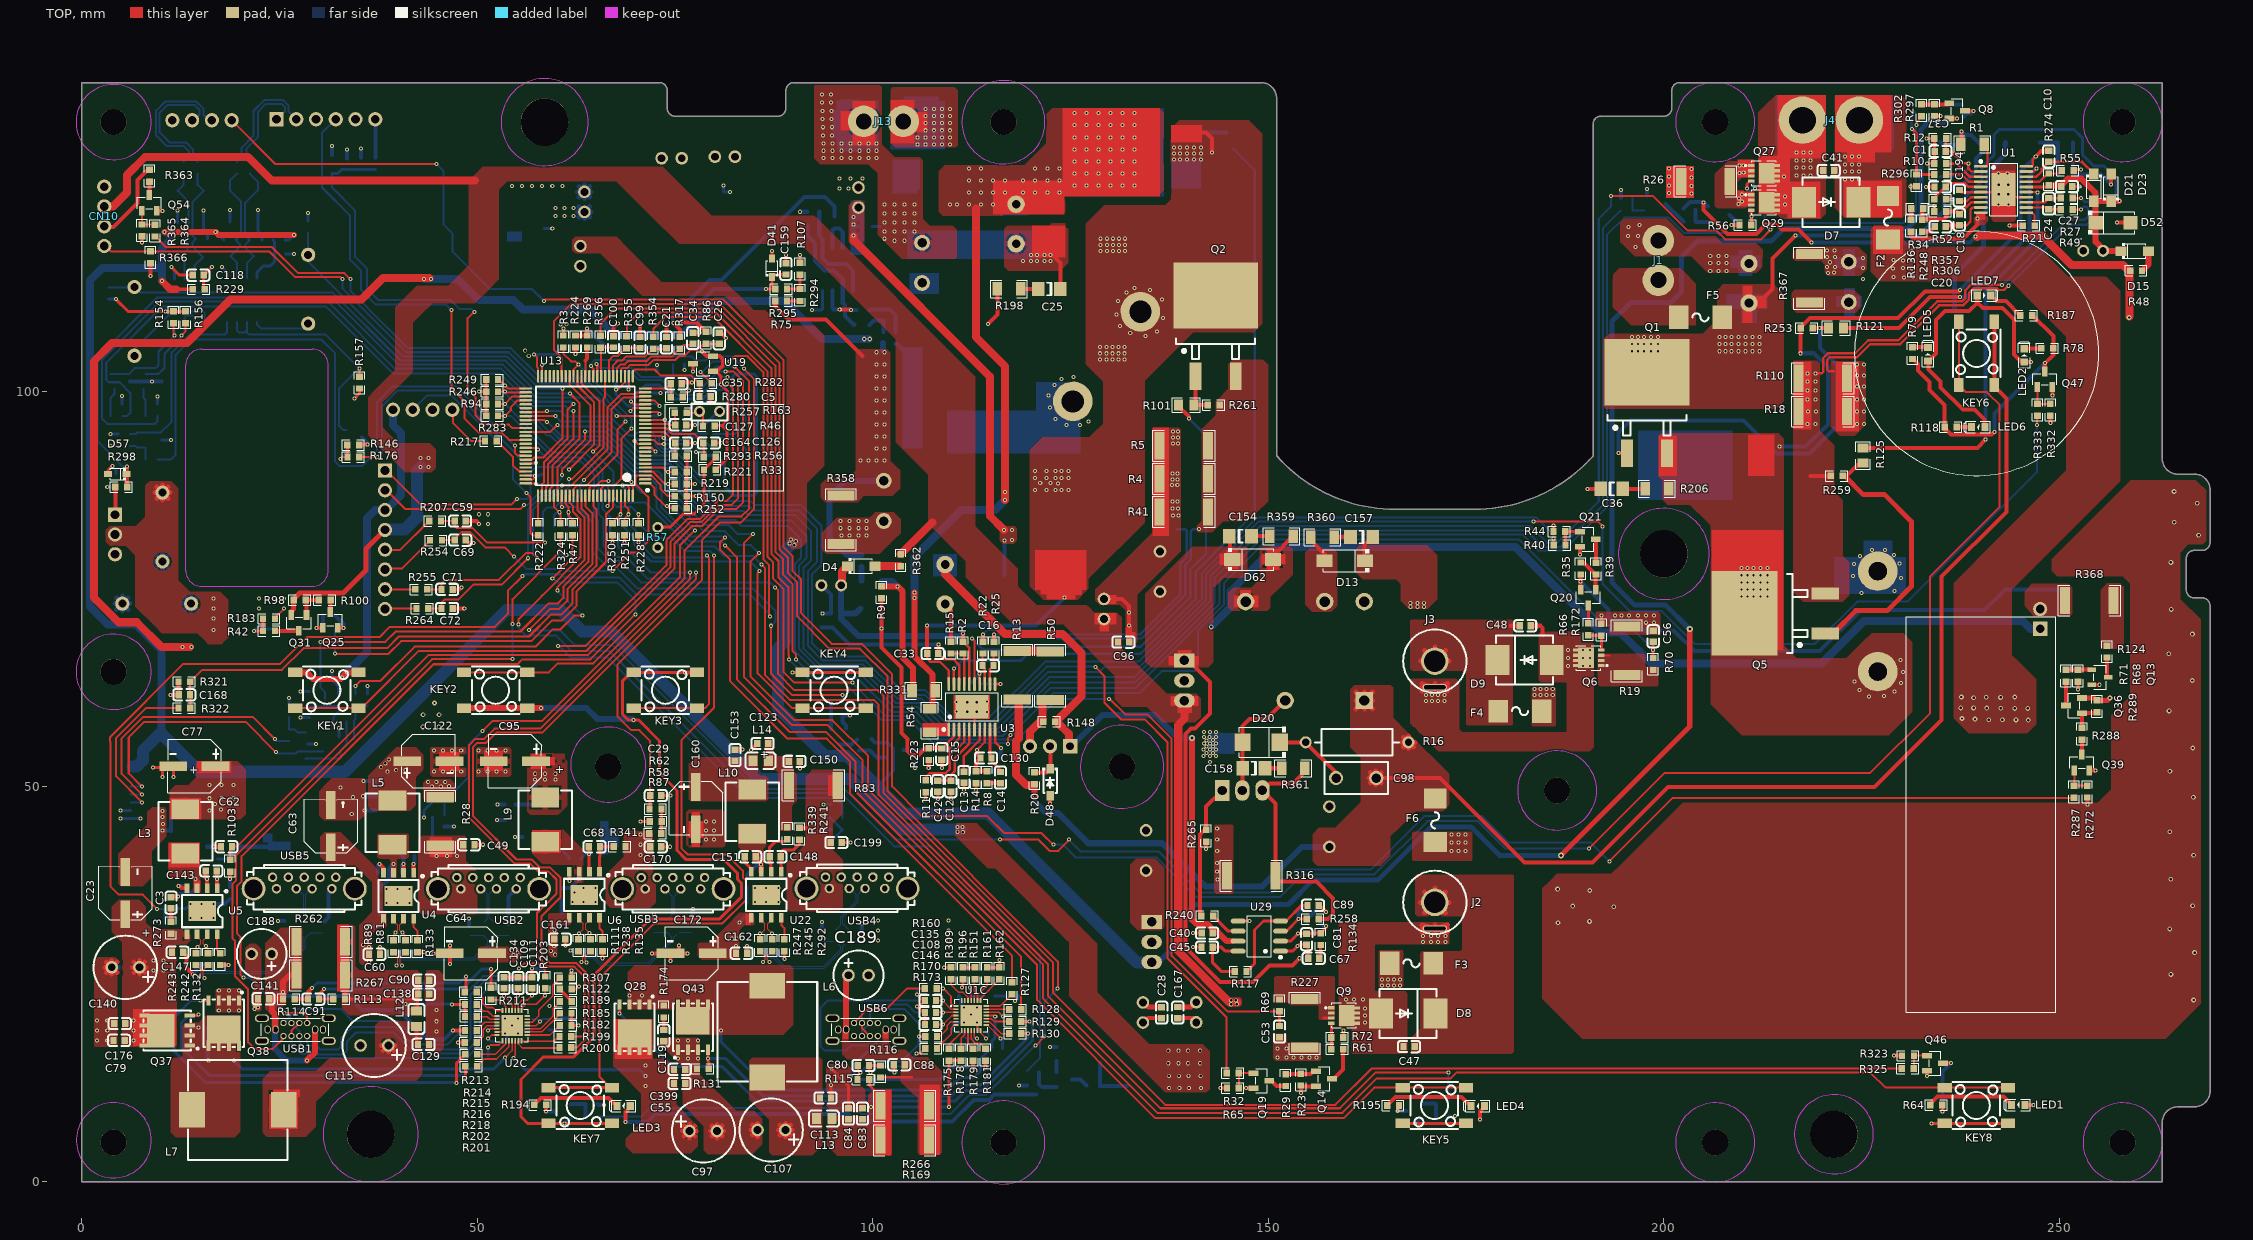
[diagram p0: TOP view]
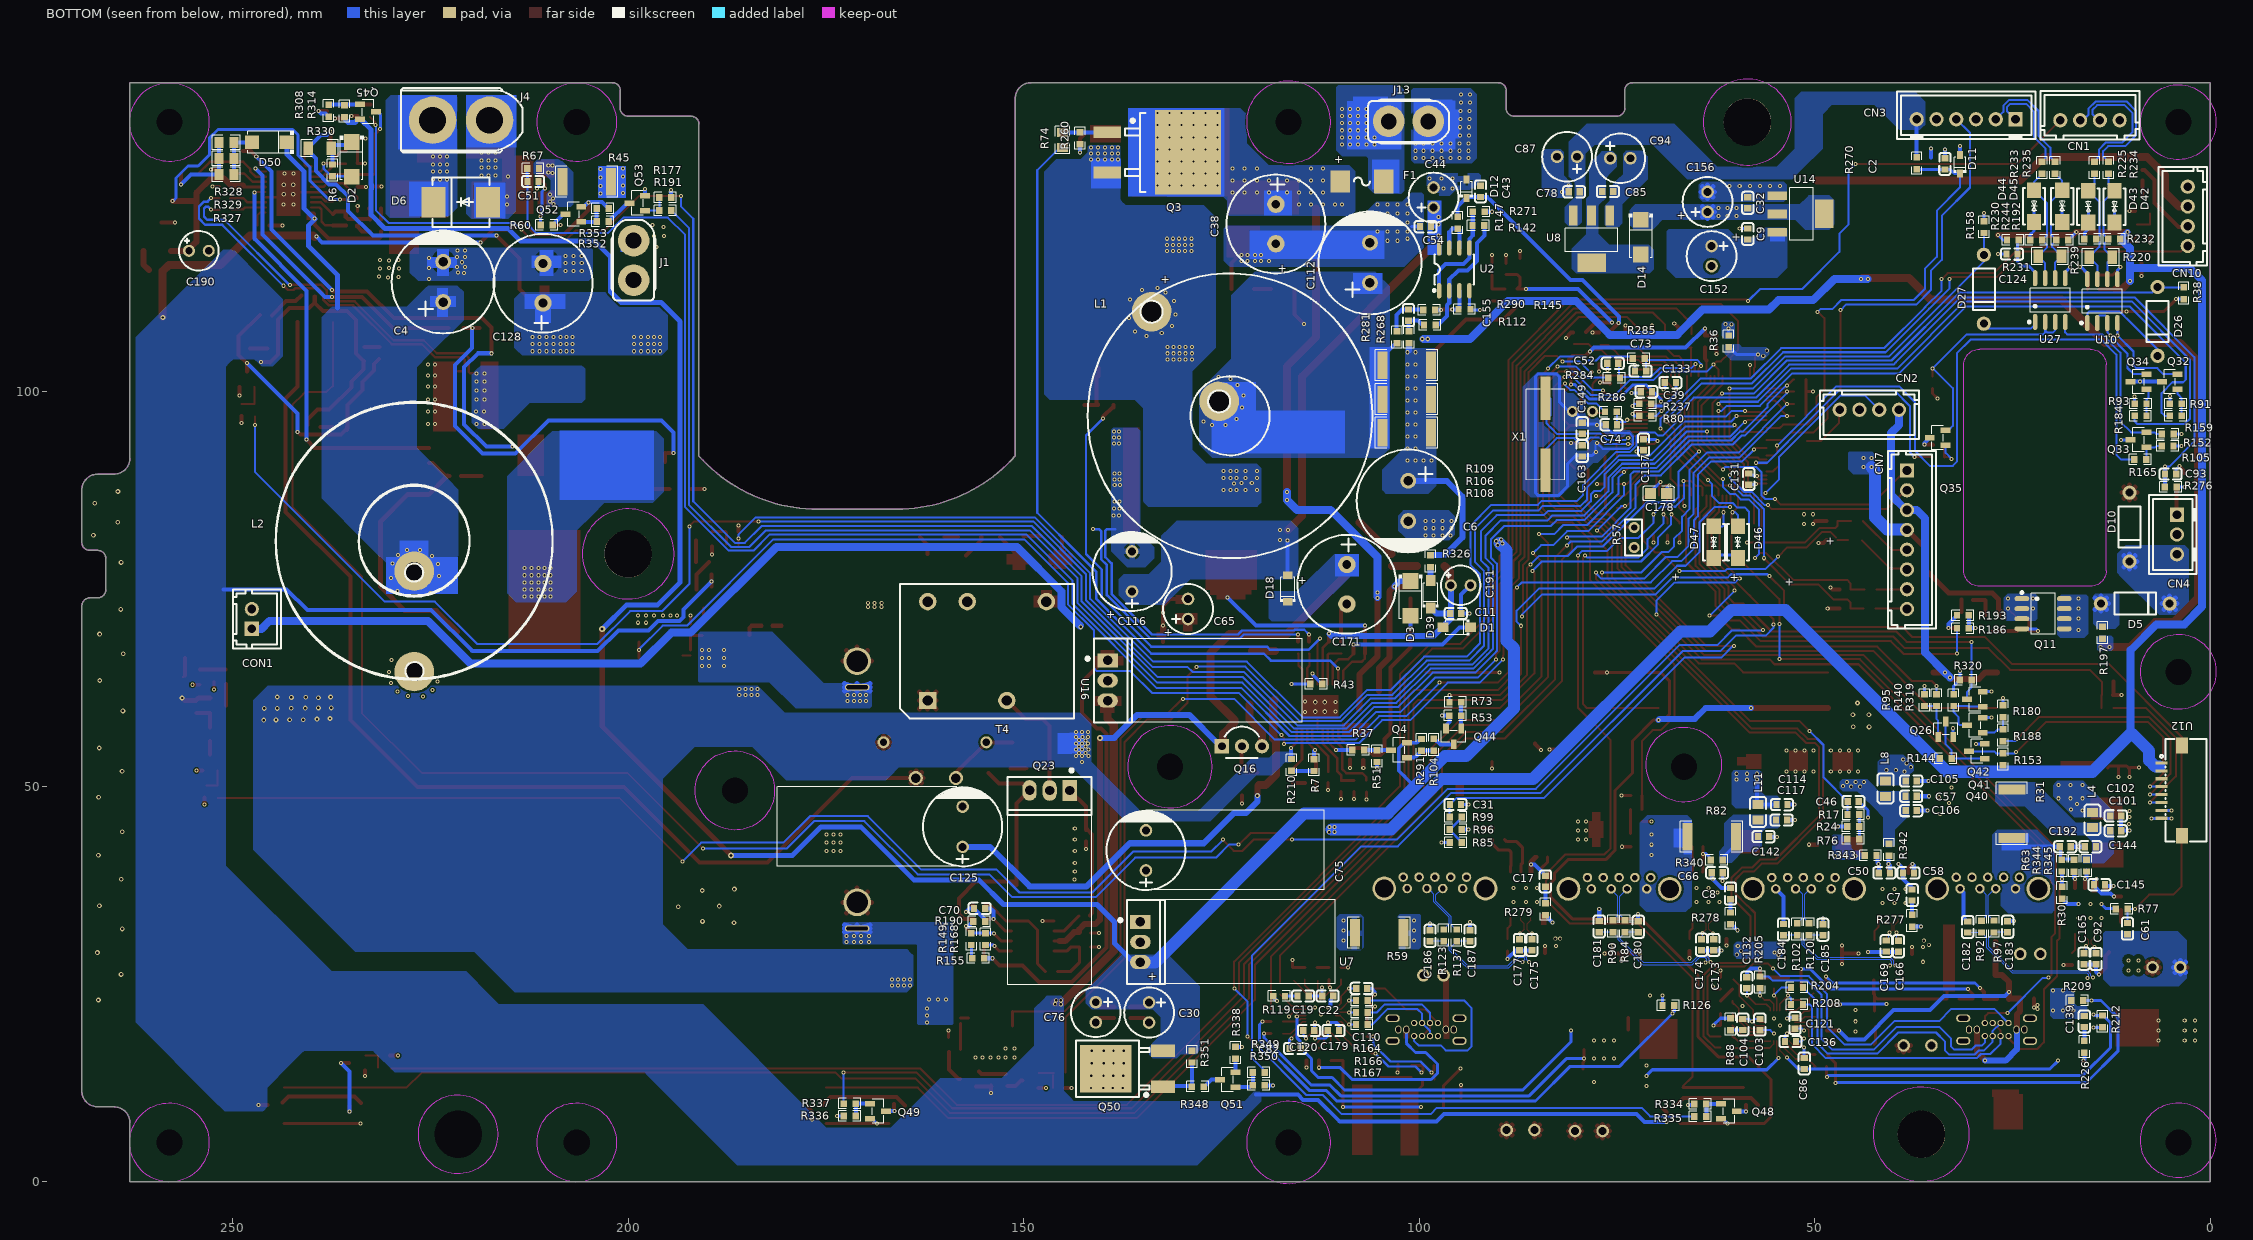
[diagram p1: BOTTOM view, seen from below]
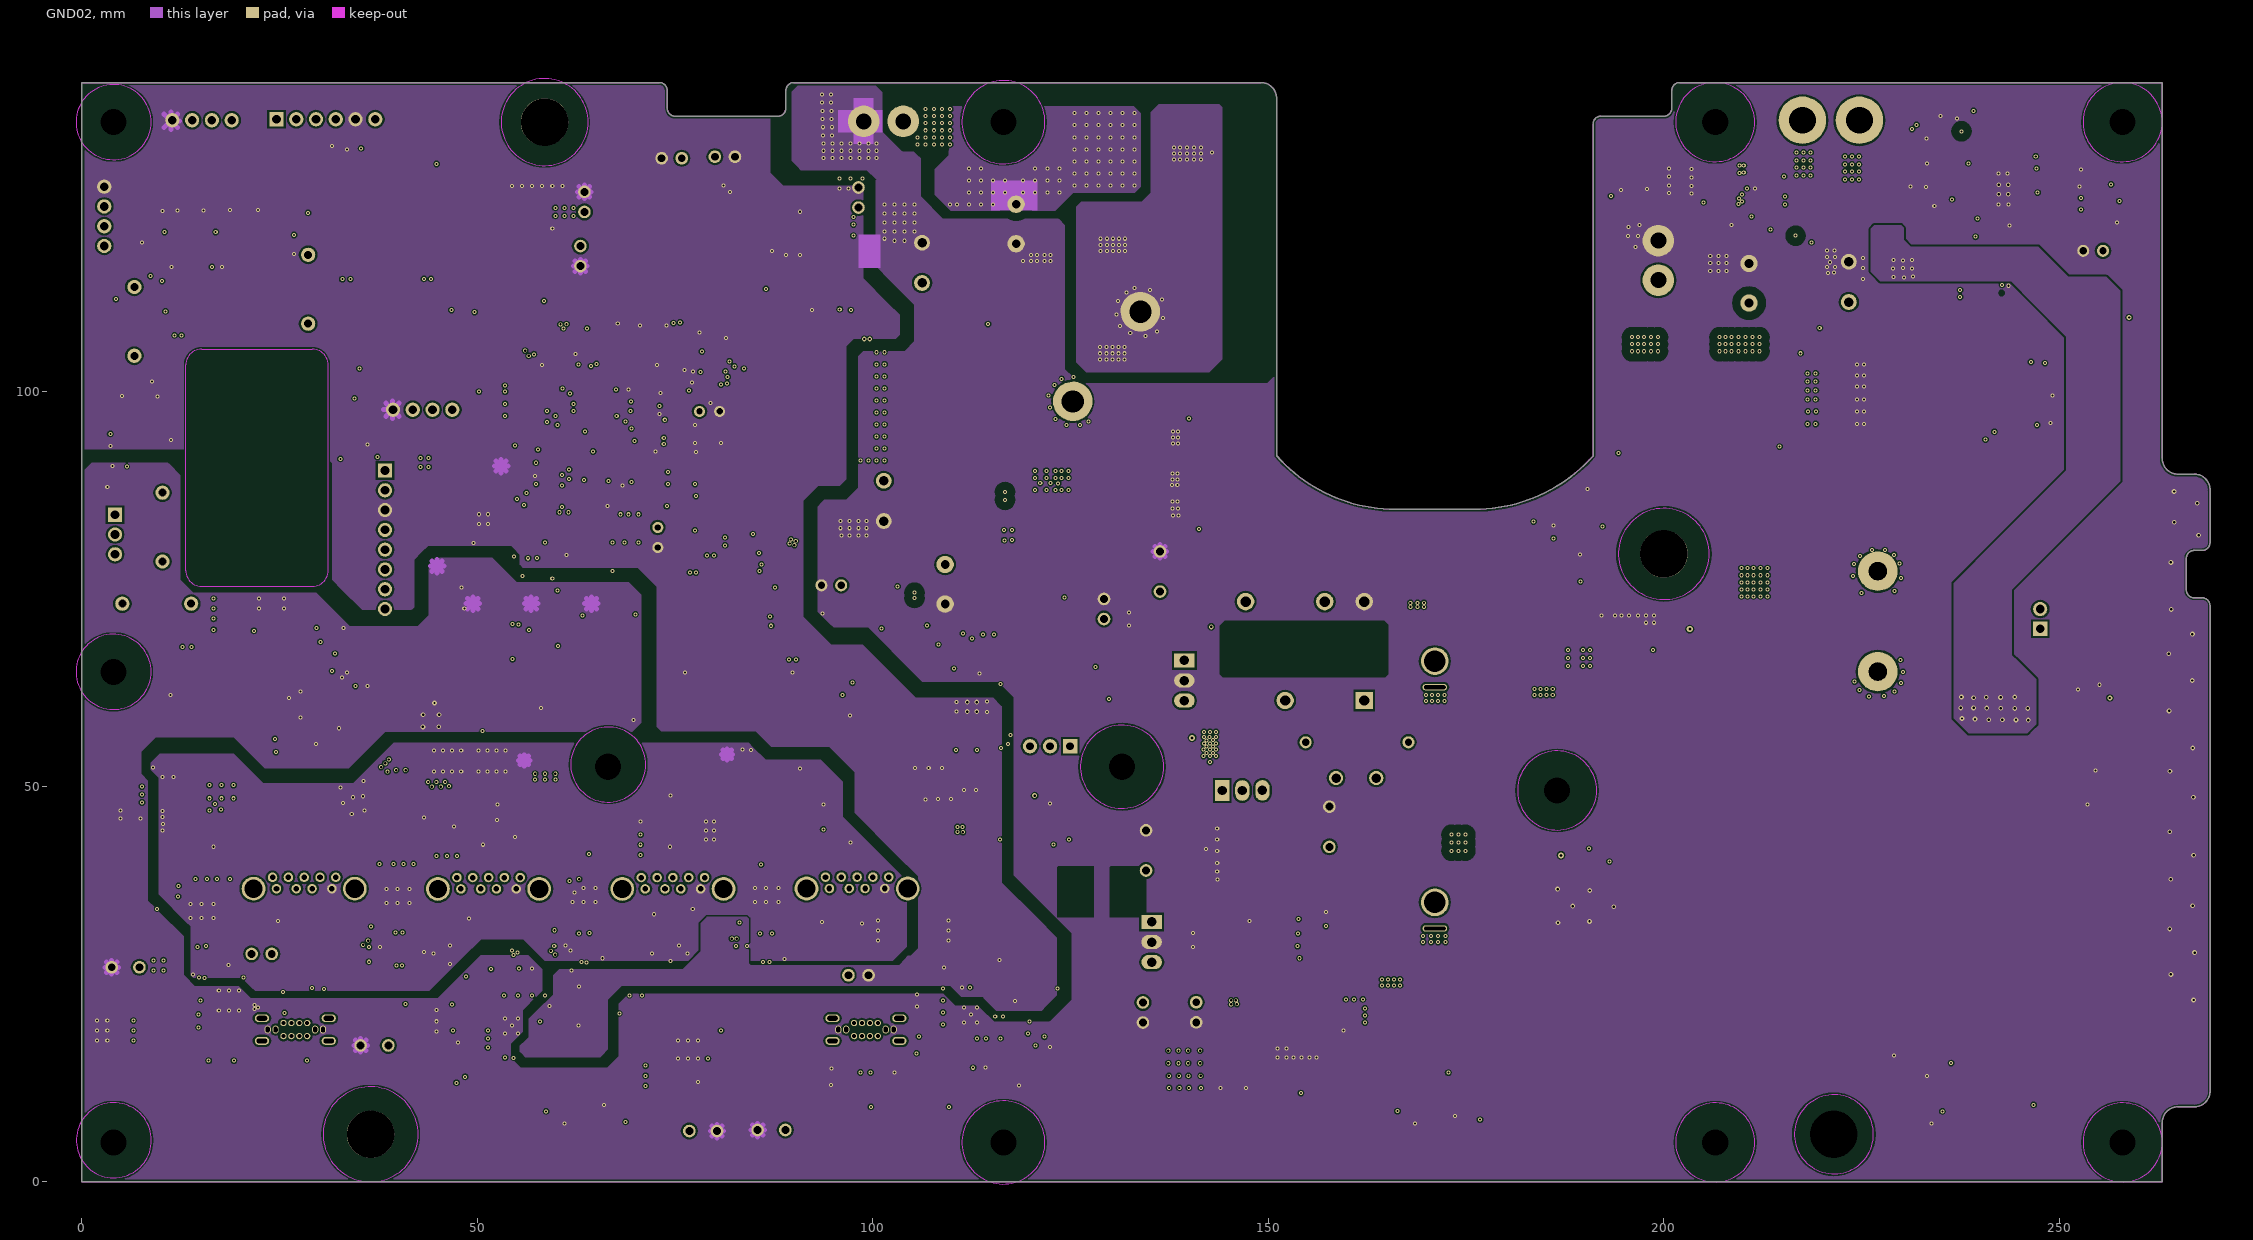
[diagram p2: GND02]
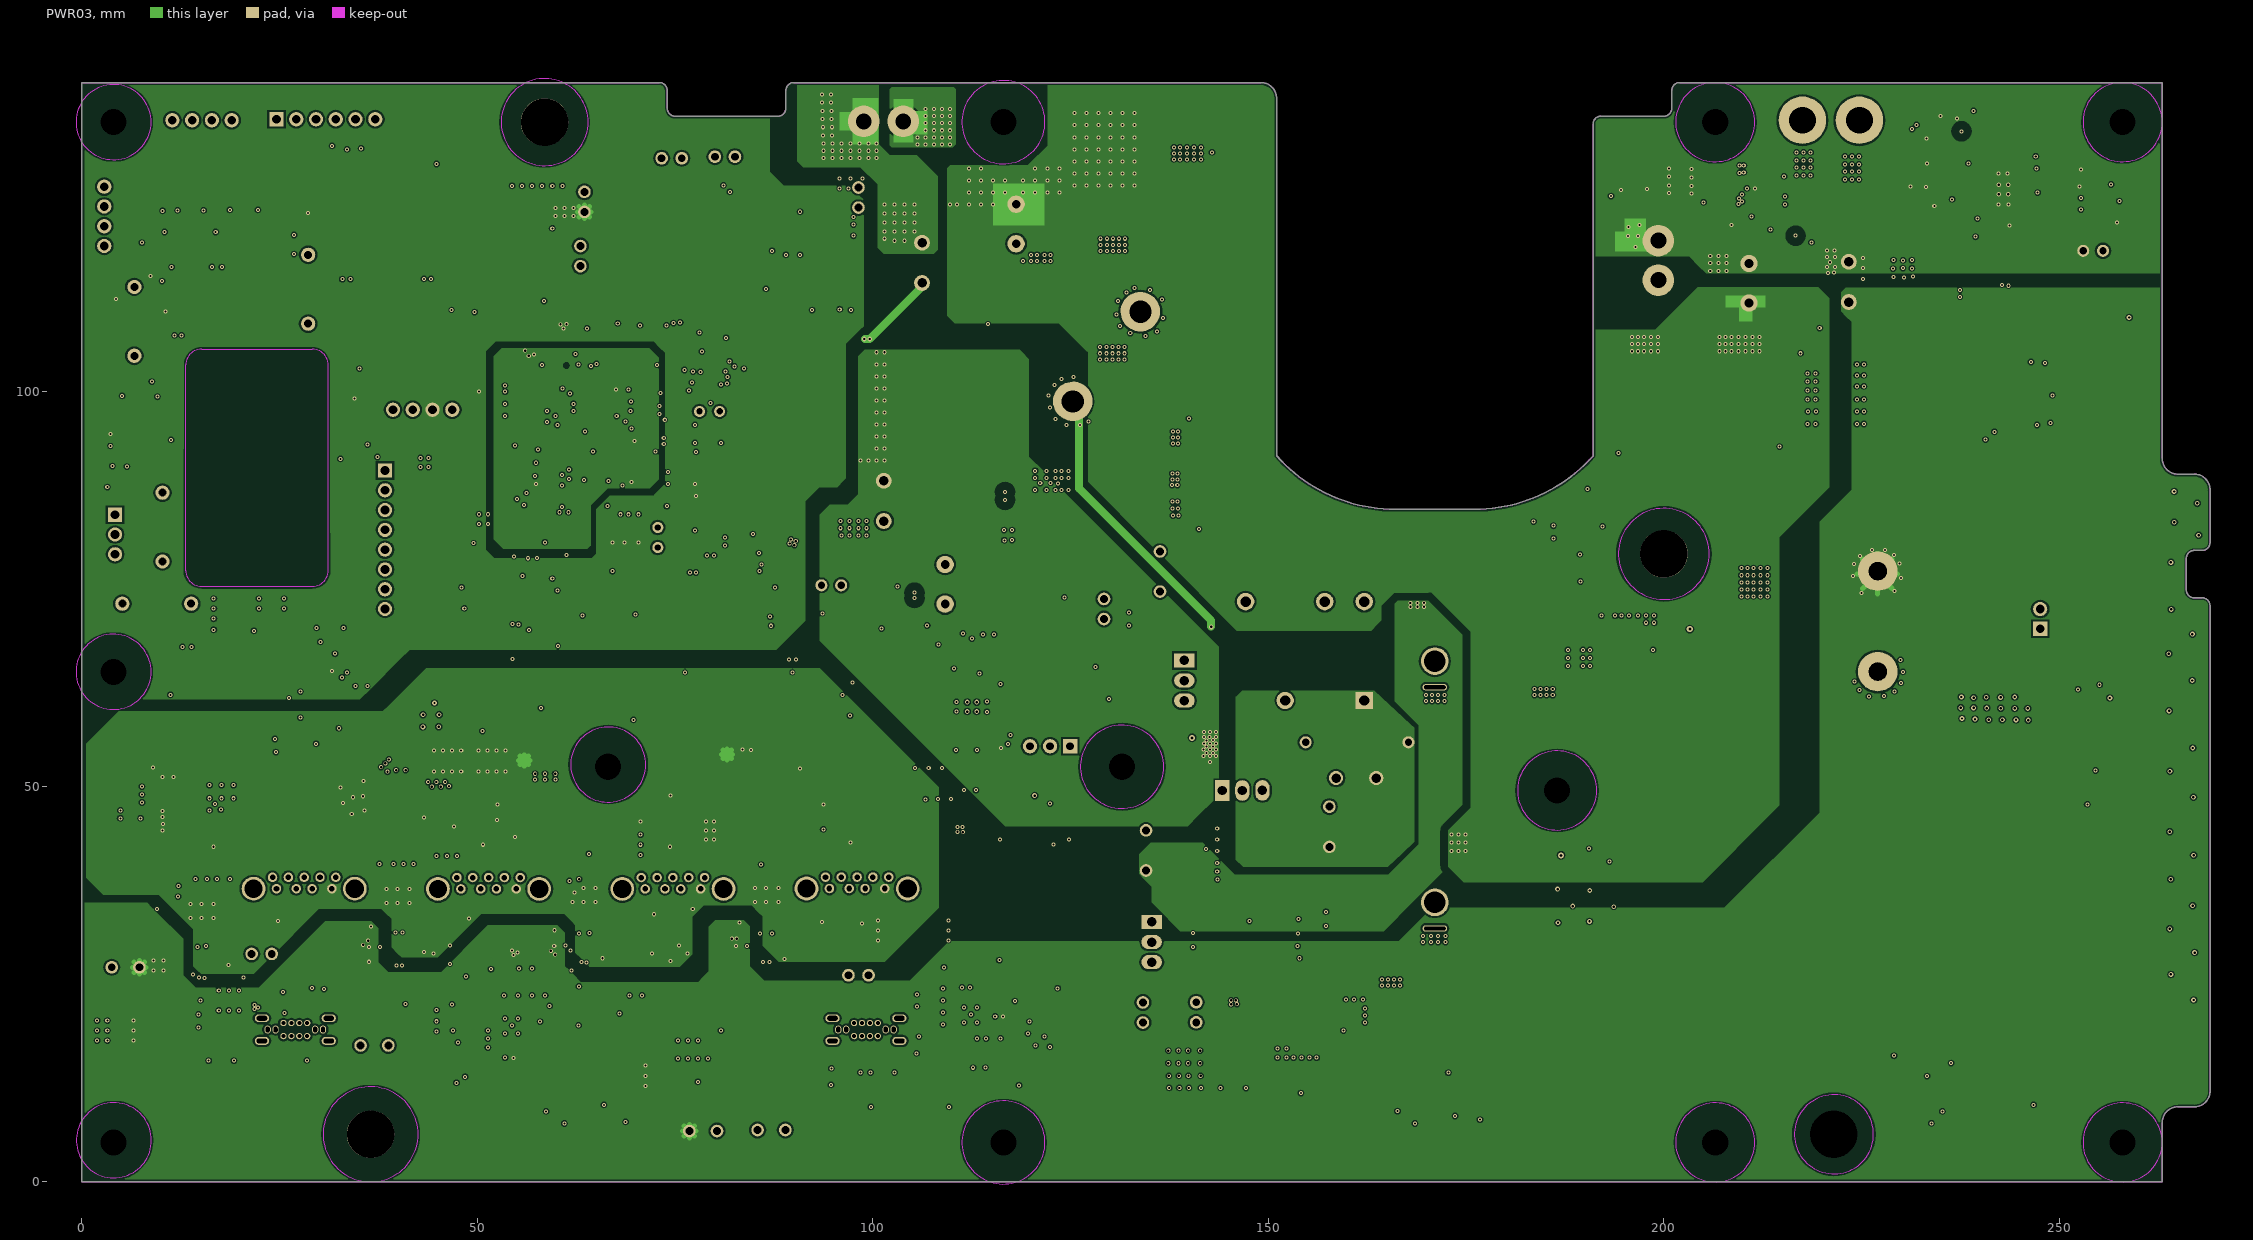
[diagram p3: PWR03]
# Altium PCB MISC84402.PcbDoc (part 1 of 12)
Units mm, origin at the board's own origin, x right, y up, seen from the top; angles counter-clockwise.
Board outline 269.06 x 139 mm, 4 copper layers (TOP, GND02, PWR03, BOTTOM), stack 0.732 mm thick; 694 components, 428 nets, 1859 pads, 1384 vias.

## Layer stack, top to bottom
TOP: signal copper 0.0305
Dielectric: core 0.2032, FR-4, Dk 4.5
GND02: signal copper 0.0305
Dielectric: core 0.2032, FR-4, Dk 4.5
PWR03: signal copper 0.0305
Dielectric: core 0.2032, FR-4, Dk 4.5
BOTTOM: signal copper 0.0305

## Board outline
75,134.75 88,134.75 ccw(c88,135.75) 89,135.75 89,138 cw(c90,138) 90,139 149.05,139 cw(c149.05,137) 151.05,137 151.05,91.821 ccw(c166.081,105.12) 166.081,85.05 176.029,85.05 ccw(c176.029,105.167) 191.049,91.785 191.05,91.785 191.05,133.75 cw(c192.05,133.75) 192.05,134.75 200,134.75 ccw(c200,135.75) 201,135.75 201,138 cw(c202,138) 202,139 263,139 263,91.5 ccw(c265,91.5) 265,89.5 267.058,89.5 cw(c267.058,87.5) 269.058,87.5 269.058,80.85 cw(c268.058,80.85) 268.058,79.85 267.058,79.85 ccw(c267.058,78.85) 266.058,78.85 266.058,74.85 ccw(c267.058,74.85) 267.058,73.85 268.058,73.85 cw(c268.058,72.85) 269.058,72.85 269.058,11.5 cw(c267.058,11.5) 267.058,9.5 265,9.5 ccw(c265,7.5) 263,7.5 263,0 0,0 0,139 73,139 cw(c73,138) 74,138 74,135.75 ccw(c75,135.75)
cut-out: -359.604,-954.134 -359.35,-954.134 -359.35,-953.88 -359.604,-953.88

## Design rules (kind name [scope] priority, off if disabled: settings)
Clearance Clearance_4 [All] p1 off: gap=1.016
Clearance Clearance_3 [InNet('B+') vs InPolygon] p2: gap=1.016
Clearance Clearance_2 [inpoly vs isvia] p3: gap=0.152
Clearance Clearance_1 [inpoly] p4: gap=0.254
Clearance [All] p5: gap=0.127
ComponentClearance [All] p1 off: gap=0.254 collisioncheckmode=3 verticalgap=0.254 showdistances=FALSE
FabricationTestPointUsage TestPointUsage [All] p1: valid=0 allowmultiple=FALSE
FabricationTestpoint Testpoint [(IsPad And (OnTopLayer Or OnBottomLayer))] p1: side=3 testpointundercomponent=TRUE minsize=1.016 maxsize=2.54 preferedsize=1.524 minholesize=0 maxholesize=1.016 preferedholesize=0.813 testpointgrid=0.025 allowsidetop=TRUE allowsidebottom=TRUE usegrid=TRUE gridtolerance=0
Height [All] p1 off: minheight=0 maxheight=25.4 prefheight=12.7
HoleSize [All] p1 off: absolutevalues=TRUE maxlimit=2.54 minlimit=0.025 maxpercent=80.000 minpercent=20.000
HoleToHoleClearance [All] p1 off: gap=0.254 allowstackedmicrovias=TRUE
LayerPairs [All] p1 off: enforce=TRUE
MinimumSolderMaskSliver [All] p1 off: minsoldermaskwidth=0
NetAntennae [All] p1: netantennaetolerance=0.025
PasteMaskExpansion [All] p1 off: expansion=0
PlaneClearance [All] p1: clearance=0.305
PlaneConnect PlaneConnect_via [isvia] p1: planeconnectstyle=Direct reliefexpansion=0.508 reliefentries=4 reliefconductorwidth=0.254 reliefairgap=0.254
PlaneConnect [All] p2: planeconnectstyle=Direct reliefexpansion=0.203 reliefentries=4 reliefconductorwidth=0.203 reliefairgap=0.203
PolygonConnect PolygonConnect_1 [isvia] p1: connectstyle=Direct reliefconductorwidth=0.254 reliefentries=4 polygonreliefangle="90 Angle"
PolygonConnect [All] p2: connectstyle=Direct reliefconductorwidth=0.762 reliefentries=4 polygonreliefangle="90 Angle"
RoutingVias [All] p1: holewidth=0.254 width=0.508 viastyle="Through Hole" minholewidth=0.254 minwidth=0.508 maxholewidth=0.254 maxwidth=0.508
SilkToSilkClearance [All] p1 off: silktosilkclearance=0
SilkscreenOverComponentPads [All] p1: minsilkscreentomaskgap=0
SolderMaskExpansion [All] p1 off: expansion=0.064
Width [All] p1: maxlimit=5.08 minlimit=0.127 preferedwidth=0.254
14 further rules are at their usual default settings.

## Classes and differential pairs
component class 屏幕电路: C168 Q26 Q40 Q41 Q42 R95 R140 R144 R153 R180 R188 R319 R320 R321 R322 U12
component class RS485: C5 C9 C21 C26 C32 C34 C35 C39 C52 C59 C69 C71 C72 C73 C74 C76 C78 C85 C87 C94 C99 C100 C126 C127 C131 C133 C137 C149 C152 C156 C163 C164 C167 C178 CN2 CN7 CN10 D14 D46 D47 KEY1 KEY2 KEY3 KEY4 KEY5 KEY7 KEY8 LED1 LED2 LED3 LED4 LED5 LED6 LED7 Q17 Q46 Q47 Q48 Q49 Q50 Q51 Q54 R3 R33 R36 R46 R47 R57 R64 R78 R79 R80 R86 R94 R118 R150 R163 R187 R194 R195 R207 R217 R219 R221 R222 R224 R228 R237 R246 R249 R250 R251 R252 R254 R255 R256 R257 R264 R269 R280 R282 R283 R284 R285 R286 R293 R317 R323 R324 R325 R332 R333 R334 R335 R336 R337 R338 R348 R349 R350 R351 R354 R355 R356 R363 R364 R365 R366 U8 U13 U14 U19 X1
component class 控制: C28 C30 C40 C45 C65 C67 C70 C75 C81 C89 C96 C98 C116 C125 C154 C157 C158 C171 D13 D18 D20 D48 D62 F6 KEY6 Q16 Q23 R13 R16 R20 R50 R117 R134 R148 R149 R155 R168 R190 R240 R258 R265 R316 R359 R360 R361 T4 U7 U16 U29
component class 降压电路: C1 C4 C6 C10 C11 C12 C13 C14 C15 C16 C18 C20 C24 C25 C27 C33 C36 C37 C38 C42 C43 C44 C54 C112 C128 C130 C155 C159 C190 C191 C194 D1 D2 D3 D4 D12 D15 D21 D23 D39 D41 D50 D52 F1 F5 J1 J13 L1 L2 Q1 Q2 Q3 Q4 Q5 Q8 Q44 Q45 R1 R2 R4 R5 R6 R7 R8 R9 R10 R11 R12 R14 R15 R18 R21 R22 R25 R27 R34 R37 R41 R43 R48 R49 R51 R52 R53 R54 R55 R73 R74 R75 R101 R104 R106 R107 R108 R109 R110 R112 R121 R125 R136 R142 R145 R147 R198 R206 R210 R223 R248 R253 R259 R260 R261 R268 R271 R274 R281 R290 R291 R294 R295 R296 R297 R302 R306 R308 R314 R326 R327 R328 R329 R330 R331 R357 R358 R362 R367 U1 U2 U3
component class 各接口: C41 C47 C48 C51 C53 C56 C93 CN4 CON1 D5 D6 D7 D8 D9 D10 D57 F2 F3 F4 J2 J3 J4 Q6 Q9 Q11 Q13 Q14 Q19 Q20 Q21 Q25 Q27 Q29 Q31 Q36 Q39 Q52 Q53 R19 R23 R26 R29 R32 R35 R39 R40 R42 R44 R45 R56 R60 R61 R65 R66 R67 R68 R69 R70 R71 R72 R98 R100 R124 R172 R177 R183 R186 R191 R193 R197 R227 R272 R276 R287 R288 R289 R298 R352 R353 R368
component class 开机启动电路: C2 C118 C124 CN1 CN3 D11 D26 D27 D42 D43 D44 D45 Q32 Q33 Q34 Q35 R38 R91 R93 R105 R146 R152 R154 R156 R157 R158 R159 R165 R176 R184 R192 R220 R225 R229 R230 R231 R232 R233 R234 R235 R239 R244 R270 U10 U27
component class QC3.0: C3 C7 C8 C17 C23 C29 C31 C46 C49 C50 C57 C58 C60 C61 C62 C63 C64 C66 C68 C77 C92 C95 C101 C102 C105 C106 C114 C117 C122 C123 C142 C143 C144 C145 C147 C148 C150 C151 C153 C160 C161 C162 C165 C166 C169 C170 C172 C173 C174 C175 C177 C180 C181 C182 C183 C184 C185 C186 C187 C192 C199 L3 L4 L5 L8 L9 L10 L11 L14 R17 R24 R28 R30 R31 R58 R59 R62 R63 R76 R77 R81 R82 R83 R84 R85 R87 R89 R90 R92 R96 R97 R99 R102 R103 R111 R120 R123 R132 R133 R135 R137 R238 R241 R242 R243 R245 R247 R273 R277 R278 R279 R292 R339 R340 R341 R342 R343 R344 R345 U4 U5 U6 U22 USB2 USB3 USB4 USB5
component class "PD 60W": C19 C22 C55 C79 C80 C82 C83 C84 C86 C88 C90 C91 C97 C103 C104 C107 C108 C109 C110 C111 C113 C115 C119 C120 C121 C129 C132 C134 C135 C136 C138 C139 C140 C141 C146 C176 C179 C188 C189 C399 L6 L7 L12 L13 Q28 Q37 Q38 Q43 R88 R113 R114 R115 R116 R119 R122 R126 R127 R128 R129 R130 R131 R151 R160 R161 R162 R164 R166 R167 R169 R170 R173 R174 R175 R178 R179 R181 R182 R185 R189 R196 R199 R200 R201 R202 R203 R204 R205 R208 R209 R211 R212 R213 R214 R215 R216 R218 R226 R262 R266 R267 R307 R309 U1C U2C USB1 USB6

## Components (designator, comment, footprint, x,y, rotation, side; value= is the part's Value field where it differs from the comment)
C1 "100nF" C0603 234.95,130.302 r180 top
C2 "100nF" C0603 33.528,128.716 r270 bottom
C3 "220pF" C0603 11.261,35.315 r90 top
C4 "1200uF" CAP-TH_BD13.0-P5.00-D1.2-FD 223.393,113.792 r90 bottom
C5 "100nF" C0603 78.781,99.314 r0 top
C6 "1200uF" CAP-TH_BD13.0-P5.00-D1.2-FD 101.386,86.106 r270 bottom
C7 "220pF" C0603 37.66,36.28 r90 bottom
C8 "220pF" C0603 60.621,36.458 r90 bottom
C9 "100nF" C0603 58.446,119.853 r270 bottom
C10 "1uF" C0603 248.666,129.667 r270 top
C11 "100nF" C0603 95.377,71.882 r0 bottom
C12 "1nF" C0603 109.855,50.038 r90 top
C13 "15nF" C0603 111.506,51.181 r270 top
C14 "2.2nF" C0603 116.129,51.13 r90 top
C15 "100nF" C0603 108.712,54.102 r270 top
C16 "100nF" C0603 114.554,65.278 r180 top
C17 "220pF" C0603 84.039,38.015 r90 bottom
C18 "56pF" C0603 237.363,121.666 r90 top
C19 "2.2nF" C0603 114.667,23.511 r0 bottom
C20 "2.2nF" C0603 234.95,120.777 r180 top
C21 "100nF" C0603 73.889,106.121 r270 top
C22 "56pF" C0603 111.556,23.505 r180 bottom
C23 "100uF" CAP-SMD_BD6.3-L6.6-W6.6-FD 5.495,36.516 r90 top
C24 "100nF" C0603 248.666,123.698 r90 top
C25 "4.7nF" C1206 122.301,112.903 r180 top
C26 "100nF" C0603 80.568,106.67 r90 top
C27 "100nF" C0603 250.952,125.857 r180 top
C28 "100nF" C0603 136.509,21.402 r270 top
C29 "1nF" C0603 72.543,48.86 r180 top
C30 "220uF" CAP-TH_BD6.3-P2.50-D1.0-FD 134.137,21.428 r270 bottom
C31 "1nF" C0603 95.403,47.717 r0 bottom
C32 "100nF" C0603 58.446,123.79 r270 bottom
C33 "1uF" C0603 107.569,66.802 r0 top
C34 "100nF" C0603 77.232,106.688 r270 top
C35 "100nF" C0603 75.142,100.923 r180 top
C36 "4.7nF" C1206 193.404,87.63 r0 top
C37 "3.9nF" C0603 234.925,125.806 r180 top
C38 "470uF" CAP-TH_BD12.5-P5.00-D0.6-FD 118.11,121.118 r270 bottom
C39 "1nF" C0603 71.257,99.914 r180 bottom
C40 "100nF" C0603 142.266,31.461 r0 top
C41 "10uF" C0603 220.853,127.889 r0 top
C42 "680pF" C0603 108.204,50.038 r90 top
C43 "1nF" C0603 92.227,125.24 r270 bottom
C44 "220uF" CAP-TH_BD6.3-P2.50-D1.0-FD 98.171,124.46 r90 bottom
C45 "100nF" C0603 142.25,29.683 r180 top
C46 "1nF" C0603 45.111,48.098 r0 bottom
C47 "10uF" C0603 167.793,17.11 r0 top
C48 "10uF" C0603 182.463,70.323 r180 top
C49 "10uF" C0603 48.921,42.637 r180 top
C50 "100nF" C0603 41.174,39.081 r180 bottom
C51 "100nF" C0603 212.025,126.502 r0 bottom
C52 "100nF" C0603 75.531,103.514 r0 bottom
C53 "100nF" C0603 151.41,19.015 r90 top
C54 "100nF" C0603 99.187,120.777 r0 bottom
C55 "2.2uF" C0603 75.56,12.463 r180 top
C56 "100nF" C0603 198.654,68.99 r270 top
C57 "100nF" C0603 37.795,48.768 r0 bottom
C58 "100nF" C0603 38.126,39.081 r180 bottom
C59 "100nF" C0603 47.814,83.566 r180 top
C60 "100nF" C0603 36.983,28.794 r180 top
C61 "100nF" C0603 10.44,32.033 r90 bottom
C62 "1nF" C0603 18.274,42.383 r0 top
C63 "100uF" CAP-SMD_BD6.3-L6.6-W6.6-FD 31.481,44.983 r90 top
C64 "100uF" CAP-SMD_BD6.3-L6.6-W6.6-FD 49.175,28.915 r180 top
C65 "220uF" CAP-TH_BD6.3-P2.50-D1.0-FD 129.218,72.441 r90 bottom
C66 "100nF" C0603 62.321,39.093 r180 bottom
C67 "100nF" C0603 155.728,28.286 r180 top
C68 "100nF" C0603 64.796,42.383 r180 top
C69 "100nF" C0603 47.817,81.153 r180 top
C70 "470pF" C0603 155.572,34.595 r0 bottom
C71 "100nF" C0603 46.166,74.93 r180 top
C72 "100nF" C0603 46.166,72.517 r180 top
C73 "100nF" C0603 72.001,102.524 r0 bottom
C74 "100nF" C0603 75.684,95.742 r0 bottom
C75 "680uF" CAP-TH_BD10.0-P5.00-D1.0-FD 134.535,41.919 r90 bottom
C76 "220uF" CAP-TH_BD6.3-P2.50-D1.0-FD 140.877,21.454 r270 bottom
C77 "100uF" CAP-SMD_BD6.3-L6.6-W6.6-FD 14.224,52.578 r180 top
C78 "100nF" C0603 80.399,125.187 r180 bottom
C79 "2.2uF" C0603 4.699,17.907 r0 top
C80 "100nF" C0603 98.806,14.732 r180 top
C81 "1nF" C0603 154.839,30.699 r90 top
C82 "100nF" C0603 115.657,16.881 r180 bottom
C83 "100nF" C0603 98.679,8.636 r270 top
C84 "100nF" C0603 96.901,8.636 r270 top
C85 "100nF" C0603 76.141,125.231 r0 bottom
C86 "100nF" C0603 51.308,14.975 r270 bottom
C87 "220uF" CAP-TH_BD6.3-P2.50-D1.0-FD 81.289,129.625 r0 bottom
C88 "10uF" C0603 103.339,14.824 r0 top
C89 "1nF" C0603 155.654,34.976 r0 top
C90 "100nF" C0603 43.219,25.502 r180 top
C91 "100nF" C0603 29.272,23.114 r0 top
C92 "10nF" C0603 14.412,28.22 r90 bottom
C93 "100nF" C0603 4.994,89.5 r0 bottom
C94 "220uF" CAP-TH_BD6.3-P2.50-D1.0-FD 74.565,129.43 r180 bottom
C95 "100uF" CAP-SMD_BD6.3-L6.6-W6.6-FD 54.737,53.213 r180 top
C96 "100nF" C0603 131.693,68.25 r0 top
C97 "220uF" CAP-TH_BD8.0-P3.50-D0.6-FD 78.54,6.442 r0 top
C98 "10nF" CAP-TH_L8.0-W4.0-P5.00-D1.2 161.096,51.071 r0 top
C99 "100nF" C0603 70.552,106.13 r270 top
C100 "100nF" C0603 67.199,106.206 r270 top
C101 "100nF" C0603 11.93,44.408 r0 bottom
C102 "10uF" C0603 11.93,46.288 r0 bottom
C103 "56pF" C0603 56.922,19.904 r90 bottom
C104 "2.2nF" C0603 59.081,19.904 r270 bottom
C105 "10uF" C0603 37.787,50.708 r0 bottom
C106 "100nF" C0603 37.787,46.948 r0 bottom
C107 "220uF" CAP-TH_BD8.0-P3.50-D0.6-FD 87.176,6.569 r180 top
C108 "100pF" C0603 107.279,21.428 r180 top
C109 "100pF" C0603 55.144,25.175 r90 top
C110 "390pF" C0603 107.261,24.476 r180 bottom
C111 "390pF" C0603 56.922,25.175 r90 top
C112 "1200uF" CAP-TH_BD13.0-P5.00-D1.2-FD 106.212,116.205 r90 bottom
C113 "10uF" C0603 94.006,10.633 r180 top
C114 "10uF" C0603 54.119,47.71 r0 bottom
C115 "220uF" CAP-TH_BD8.0-P3.50-D0.6-FD 36.983,17.265 r180 top
C116 "680uF" CAP-TH_BD10.0-P5.00-D1.0-FD 136.297,77.181 r90 bottom
C117 "100nF" C0603 54.17,45.755 r0 bottom
C118 "100nF" C0603 14.696,114.646 r180 top
C119 "2.2nF" C0603 73.559,18.507 r90 top
C120 "1uF" C0603 113.945,19.142 r0 bottom
C121 "1uF" C0603 52.474,20.077 r270 bottom
C122 "100uF" CAP-SMD_BD6.3-L6.6-W6.6-FD 43.812,53.213 r0 top
C123 "100nF" C0603 86.072,55.439 r0 top
C124 "100nF" C0603 25.045,117.313 r0 bottom
C125 "220uF" CAP-TH_BD10.0-P5.00-D1.0-FD 157.709,44.907 r90 bottom
C126 "100nF" C0603 79.258,93.437 r180 top
C127 "100nF" C0603 75.702,95.723 r180 top
C128 "470uF" CAP-TH_BD12.5-P5.00-D0.6-FD 210.769,113.625 r90 bottom
C129 "10uF" C0603 43.18,17.399 r180 top
C130 "56pF" C0603 114.3,53.594 r180 top
C131 "100nF" C0603 58.319,88.865 r270 bottom
C132 "390pF" C0603 58.573,25.191 r90 bottom
C133 "100nF" C0603 68.225,101.057 r180 bottom
C134 "100pF" C0603 53.366,25.175 r90 top
C135 "390pF" C0603 107.279,22.952 r180 top
C136 "1uF" C0603 53.05,17.745 r180 bottom
C137 "100nF" C0603 71.628,93.218 r90 bottom
C138 "100nF" C0603 43.219,23.749 r180 top
C139 "2.2nF" C0603 15.901,20.285 r270 bottom
C140 "220uF" CAP-TH_BD8.0-P3.50-D0.6-FD 5.515,27.143 r180 top
C141 "10uF" C0603 22.962,23.165 r0 top
C142 "100nF" C0603 56.449,43.662 r0 bottom
C143 "100nF" C0603 16.347,39.335 r180 top
C144 "100nF" C0603 15.123,42.383 r180 bottom
C145 "100nF" C0603 13.98,37.582 r180 bottom
C146 "100pF" C0603 107.279,19.904 r180 top
C147 "100nF" C0603 12.091,29.048 r180 top
C148 "100nF" C0603 87.656,41.113 r180 top
C149 "20pF" C0603 79.375,95.292 r270 bottom
C150 "100nF" C0603 90.069,53.178 r180 top
C151 "100nF" C0603 84.481,41.113 r180 top
C152 "220uF" CAP-TH_BD6.3-P2.50-D1.0-FD 63.018,117.059 r270 bottom
C153 "10uF" C0603 82.566,53.958 r270 top
C154 "4.7nF" C1206 146.473,81.652 r0 top
C155 "100nF" C0603 101.346,109.601 r90 bottom
C156 "220uF" CAP-TH_BD6.3-P2.50-D1.0-FD 63.526,123.917 r90 bottom
C157 "4.7nF" C1206 161.781,81.543 r180 top
C158 "4.7nF" C1206 148.167,52.308 r180 top
C159 "100nF" C0603 89,115.443 r90 top
C160 "100uF" CAP-SMD_BD6.3-L6.6-W6.6-FD 77.614,47.26 r270 top
C161 "100nF" C0603 60.413,30.699 r180 top
C162 "100nF" C0603 83.4,28.921 r180 top
C163 "20pF" C0603 79.375,92.427 r90 bottom
C164 "20pF" C0603 75.718,93.437 r180 top
C165 "10nF" C0603 15.942,28.236 r90 bottom
C166 "10nF" C0603 39.386,29.811 r90 bottom
C167 "100nF" C0603 138.547,21.413 r270 top
C168 "100nF" C0603 12.954,61.595 r0 top
C169 "10nF" C0603 40.936,29.837 r90 bottom
C170 "10uF" C0603 72.543,42.383 r180 top
C171 "470uF" CAP-TH_BD12.5-P5.00-D0.6-FD 109.133,75.565 r270 bottom
C172 "100uF" CAP-SMD_BD6.3-L6.6-W6.6-FD 77.089,28.915 r180 top
C173 "10nF" C0603 62.754,29.989 r90 bottom
C174 "10nF" C0603 64.288,30 r90 bottom
C175 "10nF" C0603 85.741,29.989 r90 bottom
C176 "100nF" C0603 4.787,20.031 r0 top
C177 "10nF" C0603 87.29,29.983 r90 bottom
C178 "4.7uF" C0805 69.712,87.036 r180 bottom
C179 "1uF" C0603 110.835,19.142 r0 bottom
C180 "10nF" C0603 72.298,32.266 r270 bottom
C181 "10nF" C0603 77.225,32.292 r270 bottom
C182 "10nF" C0603 30.642,32.241 r270 bottom
C183 "10nF" C0603 25.587,32.266 r270 bottom
C184 "10nF" C0603 53.933,31.911 r270 bottom
C185 "10nF" C0603 48.955,31.885 r270 bottom
C186 "10nF" C0603 98.612,31.123 r270 bottom
C187 "10nF" C0603 93.583,31.123 r270 bottom
C188 "100uF" CAP-TH_BD6.3-P2.50-D1.0-FD 22.724,28.837 r180 top
C189 "100uF" CAP-TH_BD6.3-P2.50-D1.0-FD 98.18,26.138 r0 top
C190 "10uF" CAP-TH_BD5.0-P2.5-D0.5-FD 254.274,117.729 r180 bottom
C191 "10uF" CAP-TH_BD5.0-P2.5-D0.5-FD 94.742,75.438 r180 bottom
C192 "10uF" C0603 18.314,42.383 r0 bottom
C194 "15nF" C0603 237.363,124.714 r90 top
C199 "10uF" C0603 95.377,42.926 r180 top
C399 "100nF" C0603 75.56,14.241 r180 top
CN1 "HX25003-4A" CONN-TH_4P-P2.50_HX25003-4A 15.18,134.884 r0 bottom
CN2 "HX25003-4A" CONN-TH_4P-P2.50_HX25003-4A 43.079,96.993 r180 bottom
CN3 "B6B-XH-A(LF)(SN)" CONN-TH_6P-P2.50_B6B-XH-A-LF-SN 30.84,134.865 r0 bottom
CN4 "B3B-XH-A(LF)(SN)" CONN-TH_3P-P2.50_B3B-XH-A-LF-SN 4.192,81.854 r270 bottom
CN7 "HX25003-8A" CONN-TH_8P-P2.50_HX25003-8A 37.673,81.196 r90 bottom
CN10 "HX25003-4A" CONN-TH_4P-P2.50_HX25003-4A 3.464,122.089 r90 top
CON1 "HX25003-2A" CONN-TH_2P-P2.50_HX25003-2A 246.929,71.181 r90 bottom
D1 "FR107_C2760867" SOD-123FL_L2.7-W1.8-LS3.8-RD 95.25,70.104 r0 bottom
D2 "RS1MD" SMA_L4.3-W2.6-LS5.2-RD 234.95,129.286 r270 bottom
D3 "RS1MD" SMA_L4.3-W2.6-LS5.2-RD 101.092,73.796 r270 bottom
D4 "FR107_C2760867" SOD-123FL_L2.7-W1.8-LS3.8-RD 98.543,77.876 r0 top
D5 "1N4007" DO-41_BD2.4-L4.7-P8.70-D0.9-RD 9.456,73.117 r0 bottom
D6 "SS34" SMC_L7.1-W6.2-LS8.1-R-RD 221.158,123.876 r180 bottom
D7 "SS34" SMC_L7.1-W6.2-LS8.1-R-RD 221.158,123.876 r180 top
D8 "SS34" SMC_L7.1-W6.2-LS8.1-R-RD 167.672,21.301 r180 top
D9 "SS34" SMC_L7.1-W6.2-LS8.1-R-RD 182.392,66.005 r0 top
D10 "1N4007" DO-41_BD2.4-L4.7-P8.70-D0.9-RD 10.186,82.801 r90 bottom
D11 "MM3Z3V3_C123917" SOD-323_L1.8-W1.3-LS2.5-RD 31.623,128.681 r90 bottom
D12 "MM3Z3V3_C123917" SOD-323_L1.8-W1.3-LS2.5-RD 94.031,125.578 r90 bottom
D13 "RS1DG" SMA_L4.4-W2.8-LS5.4-RD 159.647,78.546 r180 top
D14 "SS12" SMA_L4.3-W2.6-LS5.2-RD 71.967,119.465 r270 bottom
D15 "FR107_C2760867" SOD-123FL_L2.7-W1.8-LS3.8-RD 259.554,117.694 r0 top
D18 "1N4148W_C909967" SOD-123_L2.8-W1.8-LS3.7-RD 116.612,75.022 r90 bottom
D20 "ES3DB" SMB_L4.6-W3.6-LS5.3-RD 149.072,55.591 r180 top
D21 "FR107_C2760867" SOD-123FL_L2.7-W1.8-LS3.8-RD 254.381,125.73 r270 top
D23 "FR107_C2760867" SOD-123FL_L2.7-W1.8-LS3.8-RD 256.54,125.73 r90 top
D26 "1N4007" DO-41_BD2.4-L4.7-P8.70-D0.9-RD 6.63,108.804 r90 bottom
D27 "1N4007" DO-41_BD2.4-L4.7-P8.70-D0.9-RD 28.601,112.868 r90 bottom
D39 "FR107_C2760867" SOD-123FL_L2.7-W1.8-LS3.8-RD 98.552,74.295 r90 bottom
D41 "MM3Z3V3_C123917" SOD-323_L1.8-W1.3-LS2.5-RD 87.249,115.57 r90 top
D42 "SMAJ30" SMA_L4.3-W2.5-LS5.0-BI 12.091,123.314 r270 bottom
D43 "SMAJ30" SMA_L4.3-W2.5-LS5.0-BI 15.393,123.314 r270 bottom
D44 "SMAJ30" SMA_L4.3-W2.5-LS5.0-BI 22.251,123.377 r270 bottom
D45 "SMAJ30" SMA_L4.3-W2.5-LS5.0-BI 18.695,123.377 r270 bottom
D46 "SMAJ30" SMA_L4.3-W2.5-LS5.0-BI 59.69,80.899 r90 bottom
D47 "SMAJ30" SMA_L4.3-W2.5-LS5.0-BI 62.738,80.899 r90 bottom
D48 "MMSZ5242B_R1_00001" SOD-123_L2.7-W1.6-LS3.7-RD-1 122.403,50.538 r270 top
D50 "1SMA4733A_C382953" SMA_L4.4-W2.6-LS5.0-RD 245.364,131.445 r0 bottom
D52 "1SMA4742A_C382772" SMA_L4.4-W2.6-LS5.0-RD 256.794,121.285 r0 top
D57 "MM3Z3V3_C123917" SOD-323_L1.8-W1.3-LS2.5-RD 4.471,89.5 r180 top
D62 "RS1DG" SMA_L4.4-W2.8-LS5.4-RD 148.006,78.705 r0 top
F1 "10A/100V" FUSE-SMD_L6.1-W2.5#1 107.232,126.492 r0 bottom
F2 "FUSE/20A" FUSE-SMD_L6.1-W2.5#1 228.346,121.92 r90 top
F3 "FUSE/5A" FUSE-SMD_L6.1-W2.5#1 168.091,27.651 r0 top
F4 "FUSE/5A" FUSE-SMD_L6.1-W2.5#1 181.807,59.528 r180 top
F5 "10A/100V" FUSE-SMD_L6.1-W2.5#2 204.629,109.322 r0 top
F6 "5A/125V" FUSE-SMD_L6.1-W2.5#1 171.095,45.729 r90 top
J1 "TJC1-2A" CONN-TH_XT30UPB-F-W 199.314,116.52 r90 top
J2 "TJC1-2A" DC5521 171.049,35.35 r0 top
J3 "TJC1-2A" DC5521 171.049,65.85 r0 top
J4 "TJC1-2A" CONN-TH_XT60UPB-F-W 221.127,134.239 r0 top
J13 "TJC1-2A" CONN-TH_XT30UPB-F-W 101.336,134.086 r180 top
KEY1 "4-1437565-2" SW-SMD_4P-L6.0-W6.0-P4.50-LS8.6 30.963,62.169 r0 top locked
KEY2 "4-1437565-2" SW-SMD_4P-L6.0-W6.0-P4.50-LS8.6 52.299,62.169 r0 top locked
KEY3 "4-1437565-2" SW-SMD_4P-L6.0-W6.0-P4.50-LS8.6 73.762,62.169 r0 top locked
KEY4 "4-1437565-2" SW-SMD_4P-L6.0-W6.0-P4.50-LS8.6 95.098,62.169 r0 top locked
KEY5 "4-1437565-2" SW-SMD_4P-L6.0-W6.0-P4.50-LS8.6 171,9.669 r0 top locked
KEY6 "4-1437565-2" SW-SMD_4P-L6.0-W6.0-P4.50-LS8.6 239.548,104.75 r90 top
KEY7 "4-1437565-2" SW-SMD_4P-L6.0-W6.0-P4.50-LS8.6 62.999,9.669 r0 top
KEY8 "4-1437565-2" SW-SMD_4P-L6.0-W6.0-P4.50-LS8.6 239.499,9.67 r0 top locked
L1 "28uH" IND-TH_CS270026-W280M-N 129.546,104.364 r233 bottom locked
L2 "56uH" IND-TH_CS270026-W560M-N 227.052,70.879 r270 bottom locked
L3 "22uH" IND-SMD_L7.1-W6.8 13.081,44.323 r90 top
L4 "BLM21PG300SN1D" L0805 14.867,45.762 r270 bottom
L5 "22uH" IND-SMD_L7.1-W6.8 39.269,45.437 r90 top
L6 "10uH" IND-SMD_L13.8-W12.6_YSPI13XX 86.665,18.998 r270 top
L7 "10uH" IND-SMD_L13.8-W12.6_YSPI13XX 19.711,9.109 r0 top
L8 "BLM21PG300SN1D" L0805 41.029,49.724 r270 bottom
L9 "22uH" IND-SMD_L7.1-W6.8 58.573,45.812 r90 top
L10 "22uH" IND-SMD_L7.1-W6.8 84.735,46.828 r90 top
L11 "BLM21PG300SN1D" L0805 57.133,46.752 r270 bottom
L12 "BLM21PG300SN1D" L0805 42.291,20.651 r90 top
L13 "BLM21PG300SN1D" L0805 93.853,8.001 r0 top
L14 "BLM21PG300SN1D" L0805 85.81,53.255 r0 top
LED1 "LED-0603_R" LED0603_RED 244.805,9.754 r180 top
LED2 "LED-0603_R" LED0603_RED 245.567,104.496 r90 top
LED3 "LED-0603_R" LED0603_RED 68.478,9.627 r180 top
LED4 "LED-0603_R" LED0603_RED 176.479,9.601 r180 top
LED5 "LED-0603_R" LED0603_RED 233.384,104.64 r90 top
LED6 "LED-0603_R" LED0603_RED 239.734,95.437 r180 top
LED7 "LED-0603_R" LED0603_RED 240.479,112.081 r0 top
Q1 "CRSS042N10N" TO-263-3_L10.2-W10.7-P5.08-LS16.2-TL 197.866,98.474 r90 top
Q2 "CRSS042N10N" TO-263-3_L10.2-W10.7-P5.08-LS16.2-TL 143.332,108.179 r90 top
Q3 "CRSS042N10N" TO-263-3_L10.2-W10.7-P5.08-LS16.2-TL 133.096,130.175 r180 bottom
Q4 "SS8550_C2762207" SOT-23-3_L2.9-W1.3-P1.90-LS2.4-BR 102.54,54.61 r180 bottom
Q5 "CRSS042N10N" TO-263-3_L10.2-W10.7-P5.08-LS16.2-TL 214.073,71.882 r180 top
Q6 "AP050N03Q" PDFN-8_L3.1-W3.1-P0.65-LS3.4-BL 190.495,66.263 r90 top
Q8 "SS8050_C2898656" SOT-23-3_L2.9-W1.3-P1.90-LS2.4-BR 237.084,135.407 r180 top
Q9 "AP050N03Q" PDFN-8_L3.1-W3.1-P0.65-LS3.4-BL 159.569,21.042 r270 top
Q11 "SM4480PRL" SOP-8_L4.9-W3.9-P1.27-LS6.0-BL 21.108,71.847 r270 bottom
Q13 "AO3400_C122850" SC-59-3_L2.9-W1.5-P0.95-LS2.5-BR 255.144,63.815 r180 top
Q14 "SS8550_C2762207" SOT-23-3_L2.9-W1.3-P1.90-LS2.4-BR 157.032,13.047 r180 top
Q16 "MPSA44" TO-92-3_L4.8-W3.7-P2.54-L 122.403,55.092 r180 bottom
Q19 "SS8050_C2898656" SOT-23-3_L2.9-W1.3-P1.90-LS2.4-BR 149.114,12.81 r180 top
Q20 "SS8550_C2762207" SOT-23-3_L2.9-W1.3-P1.90-LS2.4-BR 190.435,73.879 r90 top
Q21 "SS8050_C2898656" SOT-23-3_L2.9-W1.3-P1.90-LS2.4-BR 190.389,81.263 r180 top
Q23 "IRF640NPBF" TO-220-3_L10.0-W4.5-P2.54-L 146.711,49.5 r0 bottom
Q25 "SS8050_C2898656" SOT-23-3_L2.9-W1.3-P1.90-LS2.4-BR 31.41,71.069 r270 top
Q26 "MMBT2222A_C916372" SOT-23-3_L2.9-W1.3-P1.90-LS2.4-BR 33.427,57.242 r270 bottom
Q27 "AP050N03Q" PDFN-8_L3.1-W3.1-P0.65-LS3.4-BL 212.66,127.518 r270 top
Q28 "HSBA6040" POWERPAK-SO-8_L6.2-W5.2-P1.27-BR-EP 69.876,19.573 r90 top
Q29 "AP050N03Q" PDFN-8_L3.1-W3.1-P0.65-LS3.4-BL 212.66,123.835 r270 top
Q31 "SS8550_C2762207" SOT-23-3_L2.9-W1.3-P1.90-LS2.4-BR 27.44,70.697 r90 top
Q32 "SS8550_C2762207" SOT-23-3_L2.9-W1.3-P1.90-LS2.4-BR 5.096,101.184 r180 bottom
Q33 "SS8550_C2762207" SOT-23-3_L2.9-W1.3-P1.90-LS2.4-BR 9.043,93.818 r180 bottom
Q34 "SS8550_C2762207" SOT-23-3_L2.9-W1.3-P1.90-LS2.4-BR 9.059,101.184 r180 bottom
Q35 "SS8550_C2762207" SOT-23-3_L2.9-W1.3-P1.90-LS2.4-BR 34.433,94.107 r180 bottom
Q36 "SS8550_C2762207" SOT-23-3_L2.9-W1.3-P1.90-LS2.4-BR 251.85,60.24 r0 top
Q37 "HSBA6040" POWERPAK-SO-8_L6.2-W5.2-P1.27-BR-EP 10.757,19.142 r0 top
Q38 "HSBA6040" POWERPAK-SO-8_L6.2-W5.2-P1.27-BR-EP 17.933,20.081 r90 top
Q39 "SS8050_C2898656" SOT-23-3_L2.9-W1.3-P1.90-LS2.4-BR 252.849,53.026 r270 top
Q40 "MMBT2222A_C916372" SOT-23-3_L2.9-W1.3-P1.90-LS2.4-BR 29.49,54.448 r180 bottom
Q41 "MMBT2222A_C916372" SOT-23-3_L2.9-W1.3-P1.90-LS2.4-BR 29.74,57.75 r180 bottom
Q42 "MMBT2222A_C916372" SOT-23-3_L2.9-W1.3-P1.90-LS2.4-BR 29.74,61.052 r180 bottom
Q43 "HSBA6040" POWERPAK-SO-8_L6.2-W5.2-P1.27-BR-EP 77.242,19.586 r270 top
Q44 "SS8050_C2898656" SOT-23-3_L2.9-W1.3-P1.90-LS2.4-BR 95.648,56.346 r90 bottom
Q45 "SS8550_C2762207" SOT-23-3_L2.9-W1.3-P1.90-LS2.4-BR 232.902,135.289 r0 bottom
Q46 "SS8050_C2898656" SOT-23-3_L2.9-W1.3-P1.90-LS2.4-BR 234.28,15.02 r180 top
Q47 "SS8050_C2898656" SOT-23-3_L2.9-W1.3-P1.90-LS2.4-BR 248.175,101.489 r270 top
Q48 "SS8050_C2898656" SOT-23-3_L2.9-W1.3-P1.90-LS2.4-BR 60.842,8.924 r0 bottom
Q49 "SS8050_C2898656" SOT-23-3_L2.9-W1.3-P1.90-LS2.4-BR 168.411,8.949 r0 bottom
Q50 "HSU4103" TO-252-2_L6.6-W6.1-P4.57-LS9.9-BR 137.177,14.309 r90 bottom
Q51 "SS8050_C2898656" SOT-23-3_L2.9-W1.3-P1.90-LS2.4-BR 124.197,12.946 r180 bottom
Q52 "SS8550_C2762207" SOT-23-3_L2.9-W1.3-P1.90-LS2.4-BR 206.925,122.343 r180 bottom
Q53 "SS8050_C2898656" SOT-23-3_L2.9-W1.3-P1.90-LS2.4-BR 198.847,123.766 r180 bottom
Q54 "SS8050_C2898656" SOT-23-3_L2.9-W1.3-P1.90-LS2.4-BR 8.526,123.79 r270 top
R1 "" R1206 239.014,131.191 r180 top
R2 "NC" R0603 111.379,67.564 r90 top
R3 "" R0603 60.859,106.264 r270 top
R4 "" R2512 139.323,88.9 r0 top
R5 "" R2512 139.323,93.091 r0 top
R6 "120K" R0603 237.363,127.889 r90 bottom
R7 "" R0603 113.284,52.714 r90 bottom
R8 "27K" R0603 114.427,51.181 r270 top
R9 "120K" R0603 101.092,74.549 r90 top
R10 "" R0603 234.95,128.749 r0 top
R11 "" R0603 106.68,50.038 r90 top
R12 "" R0603 234.95,131.927 r0 top